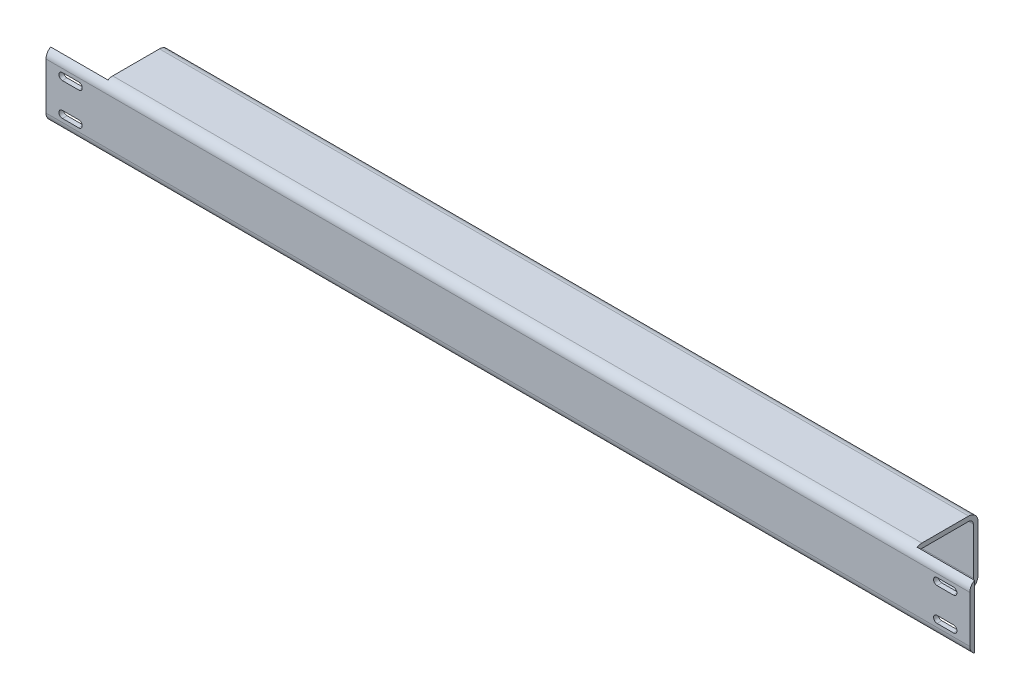
SolidWorks part; units mm, degrees
ref_plane "Front Plane" through (0, 0, 0) normal (0, 0, 1) x (1, 0, 0)
ref_plane "Top Plane" through (0, 0, 0) normal (0, 1, 0) x (1, 0, 0)
ref_plane "Right Plane" through (0, 0, 0) normal (1, 0, 0) x (0, 0, -1)
ref_plane "Plane4" through (574, 0, 0) normal (1, 0, 0) x (0, 0, -1)
sketch "Sketch1" plane through (574, 0, 0) normal (1, 0, 0) x (0, 0, -1)
  line L0 (40, -28.5714) -> (40, 28.5714)
  line L1 (28.5714, 40) -> (-28.5714, 40)
  line L2 (-40, 28.5714) -> (-40, -28.5714)
  line L3 (-28.5714, -40) -> (28.5714, -40)
  line L4 (-34.2857, -28.5714) -> (-34.2857, 28.5714)
  line L5 (-28.5714, 34.2857) -> (28.5714, 34.2857)
  line L6 (34.2857, 28.5714) -> (34.2857, -28.5714)
  line L7 (28.5714, -34.2857) -> (-28.5714, -34.2857)
  arc A0 (28.5714, -40) -> (40, -28.5714) centre (28.5714, -28.5714) ccw
  arc A1 (40, 28.5714) -> (28.5714, 40) centre (28.5714, 28.5714) ccw
  arc A2 (-28.5714, 40) -> (-40, 28.5714) centre (-28.5714, 28.5714) ccw
  arc A3 (-40, -28.5714) -> (-28.5714, -40) centre (-28.5714, -28.5714) ccw
  arc A4 (-28.5714, -34.2857) -> (-34.2857, -28.5714) centre (-28.5714, -28.5714) cw
  arc A5 (-34.2857, 28.5714) -> (-28.5714, 34.2857) centre (-28.5714, 28.5714) cw
  arc A6 (28.5714, 34.2857) -> (34.2857, 28.5714) centre (28.5714, 28.5714) cw
  arc A7 (34.2857, -28.5714) -> (28.5714, -34.2857) centre (28.5714, -28.5714) cw
  dimension "D1" = 80
extrude "Boss-Extrude1" add sketch "Sketch1" against normal blind 988
sketch "Sketch2" plane through (574, 0, 0) normal (1, 0, 0) x (0, 0, -1)
  line L0 (-34.2857, 28.5714) -> (-34.2857, 38.4689)
  line L1 (-34.2857, -28.5714) -> (-34.2857, -38.4689)
  line L2 (-34.2857, 28.5714) -> (-34.2857, -28.5714)
  line L4 (40, -28.5714) -> (40, 28.5714)
  line L5 (28.5714, 40) -> (-28.5714, 40)
  line L6 (-40, 28.5714) -> (-40, -28.5714)
  line L7 (-28.5714, -40) -> (28.5714, -40)
  line L10 (-40, 28.5714) -> (-40, -28.5714)
  arc A4 (28.5714, -40) -> (40, -28.5714) centre (28.5714, -28.5714) ccw
  arc A5 (40, 28.5714) -> (28.5714, 40) centre (28.5714, 28.5714) ccw
  arc A6 (-28.5714, 40) -> (-40, 28.5714) centre (-28.5714, 28.5714) ccw
  arc A7 (-40, -28.5714) -> (-28.5714, -40) centre (-28.5714, -28.5714) ccw
  arc A10 (-34.2857, 38.4689) -> (-40, 28.5714) centre (-28.5714, 28.5714) ccw
  arc A11 (-40, -28.5714) -> (-34.2857, -38.4689) centre (-28.5714, -28.5714) ccw
  dimension "D1" = 0
extrude "Boss-Extrude2" add sketch "Sketch2" along normal blind 70 contours L10 A11 L1 L2 L0 A10
sketch "Sketch3" plane through (-414, 0, 0) normal (-1, 0, 0) x (0, 0, 1)
  line L0 (34.2857, -28.5714) -> (34.2857, -38.4689)
  line L1 (34.2857, -28.5714) -> (34.2857, 38.4689)
  line L4 (-28.5714, -40) -> (28.5714, -40)
  line L5 (40, -28.5714) -> (40, 28.5714)
  line L6 (28.5714, 40) -> (-28.5714, 40)
  line L7 (-40, 28.5714) -> (-40, -28.5714)
  line L9 (40, -28.5714) -> (40, 28.5714)
  arc A4 (-40, -28.5714) -> (-28.5714, -40) centre (-28.5714, -28.5714) ccw
  arc A5 (28.5714, -40) -> (40, -28.5714) centre (28.5714, -28.5714) ccw
  arc A6 (40, 28.5714) -> (28.5714, 40) centre (28.5714, 28.5714) ccw
  arc A7 (-28.5714, 40) -> (-40, 28.5714) centre (-28.5714, 28.5714) ccw
  arc A9 (34.2857, -38.4689) -> (40, -28.5714) centre (28.5714, -28.5714) ccw
  arc A10 (40, 28.5714) -> (34.2857, 38.4689) centre (28.5714, 28.5714) ccw
  dimension "D1" = 0
extrude "Boss-Extrude3" add sketch "Sketch3" along normal blind 70
sketch "Sketch4" plane through (0, 0, 40) normal (0, 0, 1) x (1, 0, 0)
  line L0 (-1000, 0) -> (49000, 0) construction
  line L1 (-464, 20) -> (-444, 20) construction
  line L2 (-464, 24.25) -> (-444, 24.25)
  line L3 (-464, 15.75) -> (-444, 15.75)
  line L4 (-414, 40) -> (574, 40) construction
  line L5 (-484, -28.5714) -> (-484, 28.5714) construction
  line L6 (604, 20) -> (624, 20) construction
  line L7 (-464, -20) -> (-444, -20) construction
  line L8 (-464, -24.25) -> (-444, -24.25)
  line L9 (-464, -15.75) -> (-444, -15.75)
  line L10 (604, 24.25) -> (624, 24.25)
  line L11 (604, 15.75) -> (624, 15.75)
  line L12 (644, 28.5714) -> (644, -28.5714) construction
  line L13 (604, -20) -> (624, -20) construction
  line L14 (604, -24.25) -> (624, -24.25)
  line L15 (604, -15.75) -> (624, -15.75)
  arc A0 (-464, 24.25) -> (-464, 15.75) centre (-464, 20) ccw
  arc A1 (-444, 15.75) -> (-444, 24.25) centre (-444, 20) ccw
  arc A2 (-464, -24.25) -> (-464, -15.75) centre (-464, -20) cw
  arc A3 (-444, -15.75) -> (-444, -24.25) centre (-444, -20) cw
  arc A4 (604, 24.25) -> (604, 15.75) centre (604, 20) ccw
  arc A5 (624, 15.75) -> (624, 24.25) centre (624, 20) ccw
  arc A6 (604, -24.25) -> (604, -15.75) centre (604, -20) cw
  arc A7 (624, -15.75) -> (624, -24.25) centre (624, -20) cw
  point P5 (-454, 20)
  point P18 (-454, -20)
  point P23 (614, 20)
  point P32 (614, -20)
  dimension "D2" = 4.25
  dimension "D6" = 4.25
  dimension "D1" = 20
  dimension "D3" = 20
  dimension "D4" = 30
  dimension "D5" = 20
  dimension "D7" = 30
extrude "Cut-Extrude1" cut sketch "Sketch4" against normal blind 70
